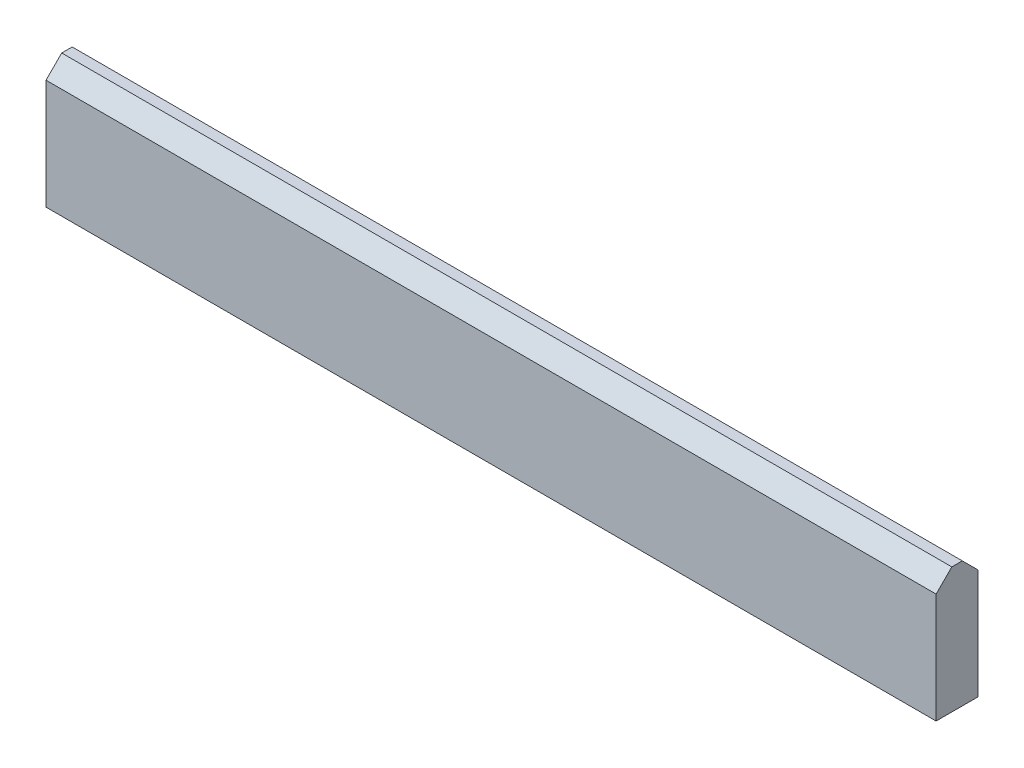
from build123d import *

# Parameters (mm, degrees)
SKETCH1_W           = 850
SKETCH1_H           = 120
BOSS_EXTRUDE1_DEPTH = 20
CHAMFER1_SIZE       = 15


with BuildPart() as part:
    # Sketch1 → Boss-Extrude1 (new, symmetric)
    with BuildSketch(Plane.XY):
        Rectangle(SKETCH1_W, SKETCH1_H)
    extrude(amount=BOSS_EXTRUDE1_DEPTH, both=True)

    # Chamfer1
    chamfer1_edges = [part.edges().sort_by_distance(p)[0] for p in [
        (0, 60, 20),
        (0, 60, -20),
    ]]
    chamfer(chamfer1_edges, length=CHAMFER1_SIZE)


solid = part.part
